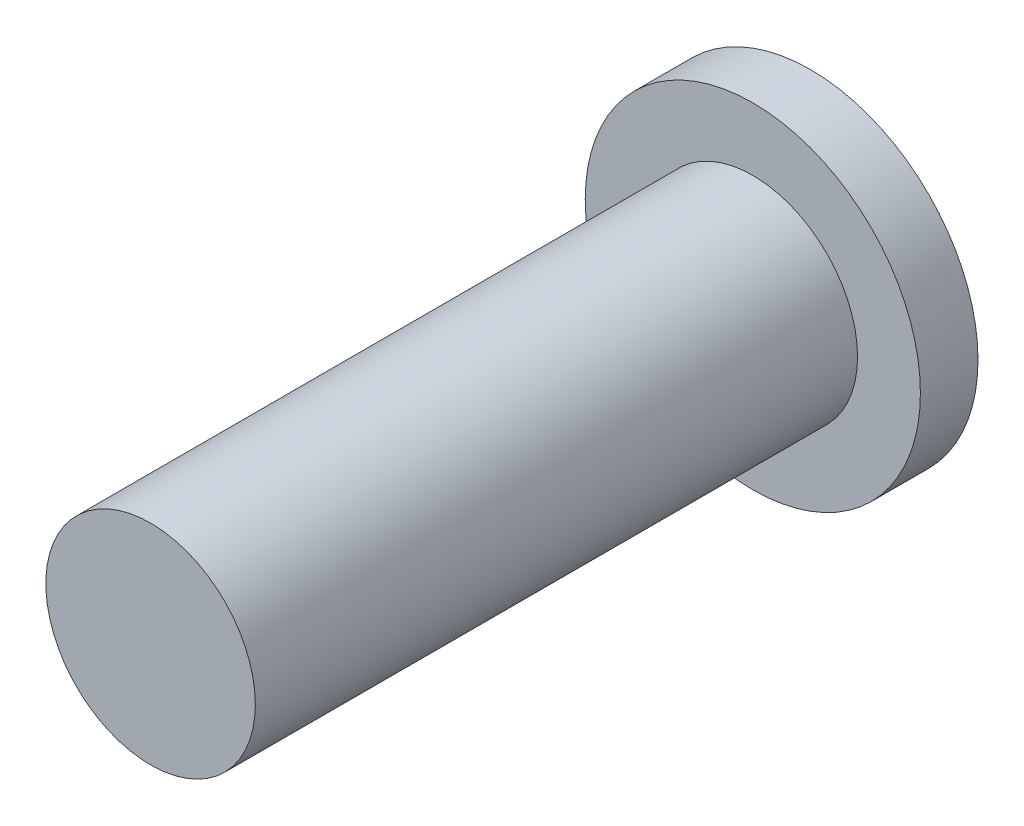
SolidWorks part; units mm, degrees
ref_plane "前视基准面" through (0, 0, 0) normal (0, 0, 1) x (1, 0, 0)
ref_plane "上视基准面" through (0, 0, 0) normal (0, 1, 0) x (1, 0, 0)
ref_plane "右视基准面" through (0, 0, 0) normal (1, 0, 0) x (0, 0, -1)
other "Configuration Table"
sketch "草图1" plane through (0, 0, 0) normal (0, 0, 1) x (1, 0, 0)
  circle A0 centre (0, 0) radius 10
  point P0 (0, 0)
  dimension "D1" = 20
extrude "凸台-拉伸1" add sketch "草图1" along normal blind 63
sketch "草图2" plane through (0, 0, 0) normal (0, 0, 1) x (1, 0, 0)
  circle A0 centre (0, 0) radius 16
  point P0 (0, 0)
  dimension "D1" = 32
extrude "凸台-拉伸2" add sketch "草图2" along normal blind 5.5
